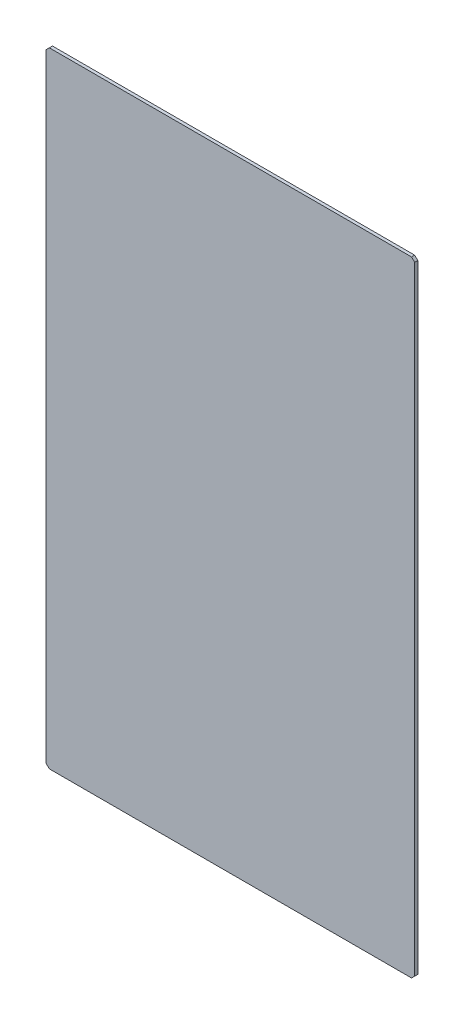
from build123d import *

# Parameters (mm, degrees)
SKETCH_1_W      = 590
SKETCH_1_H      = 1000
EXTRUDE_1_DEPTH = 5
CHAMFER_1_SIZE  = 5


with BuildPart() as part:
    # 草图1 → 拉伸1 (new body)
    with BuildSketch(Plane.XY):
        Rectangle(SKETCH_1_W, SKETCH_1_H)
    extrude(amount=EXTRUDE_1_DEPTH)

    # 倒角1
    chamfer_1_edges = [part.edges().sort_by_distance(p)[0] for p in [
        (-295, 500, 2.5),
        (295, 500, 2.5),
        (295, -500, 2.5),
        (-295, -500, 2.5),
    ]]
    chamfer(chamfer_1_edges, length=CHAMFER_1_SIZE)


solid = part.part
